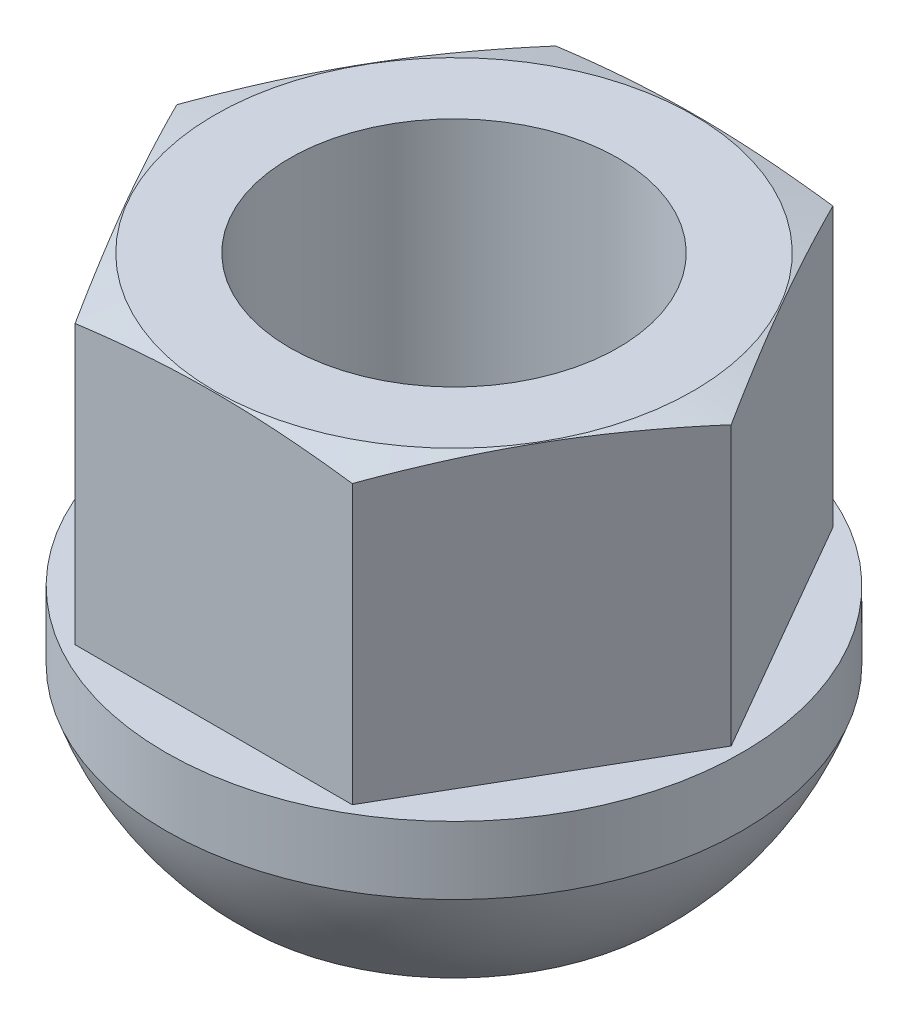
from build123d import *

# Parameters (mm, degrees)
M22X1_5_1_D         = 20.5
SKETCH_4_OUTSIDE_W  = 49.818
SKETCH_4_OUTSIDE_H  = 49.818
CUT_EXTRUDE_1_DEPTH = 18


with BuildPart() as part:
    # 草图1 → 旋转1 (revolve)
    with BuildSketch(Plane.XY, mode=Mode.PRIVATE) as revolve_1_sk:
        with BuildLine():
            Line((-18, 7.77364393), (-18, 30))
            Line((-18, 30), (-10, 30))
            Line((-10, 30), (-10, 5.2))
            Line((-10, 5.2), (-11.25, 4))
            Line((-11.25, 4), (-11.25, 0))
            Line((-11.25, 0), (-13, 0))
            ThreePointArc((-13, 0), (-15.979905663, 3.578147123), (-18, 7.77364393))
        make_face()
    revolve(revolve_1_sk.sketch.rotate(Axis((0, 29.86875, 0), (0, -1, 0)), 270), axis=Axis((0, 29.86875, 0), (0, -1, 0)))

    # M22x1.5 螺纹孔1 (through all)
    with Locations(Plane(origin=(0, 30, 0), x_dir=(1, 0, 0), z_dir=(0, 1, 0))):
        with Locations((0, 0)):
            Hole(M22X1_5_1_D / 2)

    # 草图4 outside → 切除-拉伸1 (cut)
    with BuildSketch(Plane(origin=(0, 30, 0), x_dir=(1, 0, 0), z_dir=(0, 1, 0))):
        Rectangle(SKETCH_4_OUTSIDE_W, SKETCH_4_OUTSIDE_H)
        Polygon((-8.65, 15), (8.65, 15), (17.3, 0), (8.65, -15), (-8.65, -15), (-17.3, 0), align=None, mode=Mode.SUBTRACT)
    extrude(amount=-CUT_EXTRUDE_1_DEPTH, mode=Mode.SUBTRACT)

    # 草图6 → 切除-旋转8 (revolve, cut)
    with BuildSketch(Plane(origin=(0, 0, 0), x_dir=(0, 0, -1), z_dir=(1, 0, 0)), mode=Mode.PRIVATE) as cut_revolve_8_sk:
        Polygon((6.162949371, 32.348642693), (24.147556169, 27.529681825), (24.147556169, 34), (6.162949371, 34), align=None)
    revolve(cut_revolve_8_sk.sketch.rotate(Axis((0, 32.348642693, 0), (0, 1, 0)), 90), axis=Axis((0, 32.348642693, 0), (0, 1, 0)), mode=Mode.SUBTRACT)


solid = part.part
